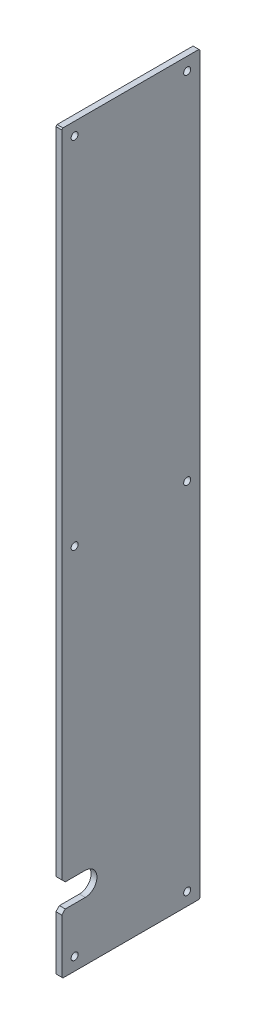
from build123d import *

# Parameters (mm, degrees)
SKETCH_1_W          = 118
SKETCH_1_H          = 628
EXTRUDE_1_DEPTH     = 5
CHAMFER_1_SIZE      = 1
SKETCH_2_R          = 3
CUT_EXTRUDE_1_DEPTH = 320.534035746
CUT_EXTRUDE_2_DEPTH = 320.534035746
CHAMFER_2_SIZE      = 3


with BuildPart() as part:
    # 草图1 → 凸台-拉伸1 (new body)
    with BuildSketch(Plane(origin=(0, 0, 0), x_dir=(0, 0, -1), z_dir=(1, 0, 0))):
        Rectangle(SKETCH_1_W, SKETCH_1_H)
    extrude(amount=EXTRUDE_1_DEPTH)

    # 倒角1
    chamfer_1_edges = [part.edges().sort_by_distance(p)[0] for p in [
        (2.5, 314, 59),
        (2.5, 314, -59),
        (2.5, -314, -59),
        (2.5, -314, 59),
    ]]
    chamfer(chamfer_1_edges, length=CHAMFER_1_SIZE)

    # 草图2 → 切除-拉伸1 (cut, through all)
    with BuildSketch(Plane.ZY):
        with Locations((-48, 303)):
            Circle(SKETCH_2_R)
        with Locations(Location((-48, -303, 0), (0, 0, 180))):
            Circle(SKETCH_2_R)
        with Locations((48, -303)):
            Circle(SKETCH_2_R)
        with Locations(Location((48, 303, 0), (0, 0, 180))):
            Circle(SKETCH_2_R)
        with Locations((48, 0)):
            Circle(SKETCH_2_R)
        with Locations((-48, 0)):
            Circle(SKETCH_2_R)
    extrude(amount=-CUT_EXTRUDE_1_DEPTH, mode=Mode.SUBTRACT)

    # 草图3 → 切除-拉伸2 (cut, through all)
    with BuildSketch(Plane(origin=(5, 0, 0), x_dir=(0, 0, -1), z_dir=(1, 0, 0))):
        with BuildLine():
            Line((-39, -264), (-59, -264))
            ThreePointArc((-59, -264), (-69, -254), (-59, -244))
            Line((-59, -244), (-39, -244))
            ThreePointArc((-39, -244), (-29, -254), (-39, -264))
        make_face()
    extrude(amount=-CUT_EXTRUDE_2_DEPTH, mode=Mode.SUBTRACT)

    # 倒角2
    chamfer_2_edges = [part.edges().sort_by_distance(p)[0] for p in [
        (2.5, -264, 59),
        (2.5, -244, 59),
    ]]
    chamfer(chamfer_2_edges, length=CHAMFER_2_SIZE)


solid = part.part
